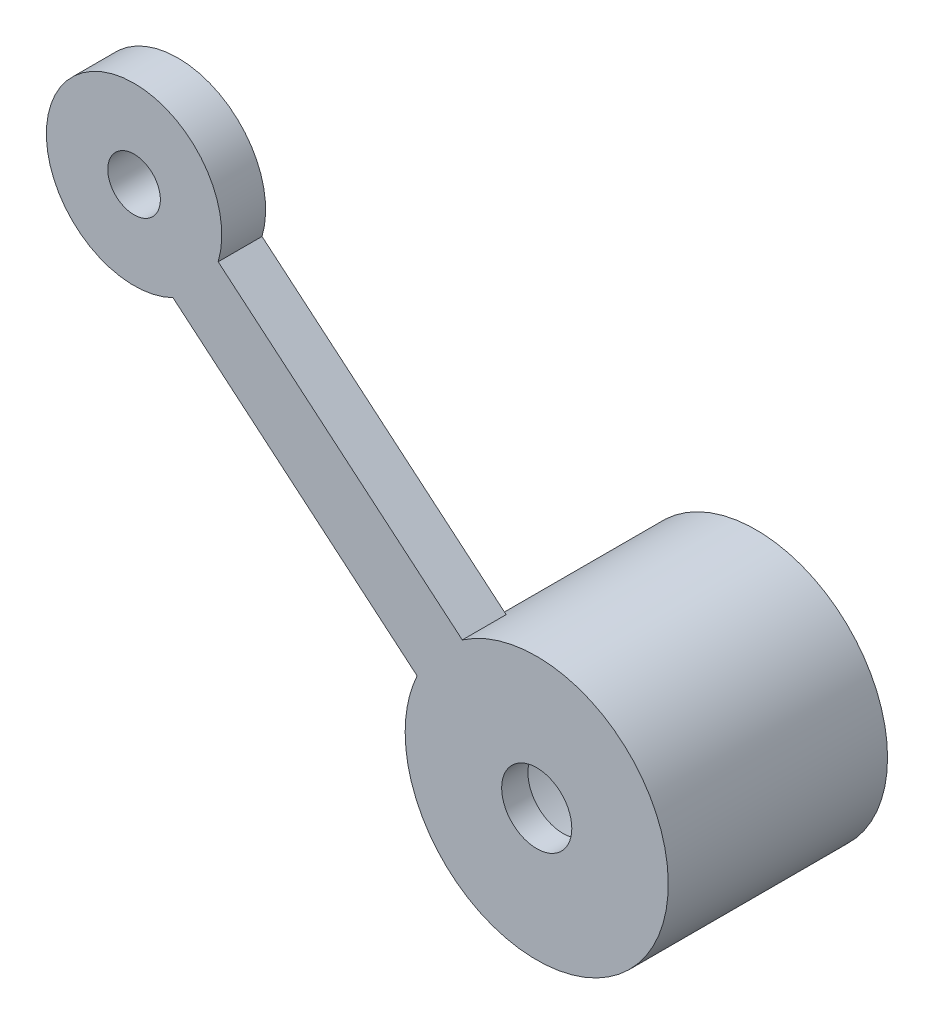
from build123d import *

# Parameters (mm, degrees)
SKETCH1_R           = 3
SKETCH1_R_2         = 4
BOSS_EXTRUDE1_DEPTH = 5
SKETCH2_R           = 13
CUT_EXTRUDE1_DEPTH  = 2
SKETCH4_R           = 1.25
BOSS_EXTRUDE2_DEPTH = 2
BOSS_EXTRUDE3_START = 20
SKETCH5_R           = 15
SKETCH5_R_2         = 13
BOSS_EXTRUDE3_DEPTH = 20


with BuildPart() as part:
    # Sketch1 → Boss-Extrude1 (new body)
    with BuildSketch(Plane.XY):
        with BuildLine():
            Line((4.437522393, -8.961495132), (32.27272364, -32.382887973))
            ThreePointArc((32.27272364, -32.382887973), (57.387408796, -48.287527496), (37.423393239, -26.261564368))
            Line((37.423393239, -26.261564368), (9.588191993, -2.840171527))
            ThreePointArc((9.588191993, -2.840171527), (-7.651654506, 6.438336999), (4.437522393, -8.961495132))
        make_face()
        Circle(SKETCH1_R, mode=Mode.SUBTRACT)
        with Locations((45.909927037, -38.630021997)):
            Circle(SKETCH1_R_2, mode=Mode.SUBTRACT)
    extrude(amount=BOSS_EXTRUDE1_DEPTH)

    # Sketch2 → Cut-Extrude1 (cut)
    with BuildSketch(Plane(origin=(0, 0, 0), x_dir=(-1, 0, 0), z_dir=(0, 0, -1))):
        with Locations((-45.909927037, -38.630021997)):
            Circle(SKETCH2_R)
    extrude(amount=-CUT_EXTRUDE1_DEPTH, mode=Mode.SUBTRACT)

    # Sketch4 → Boss-Extrude2 (add)
    with BuildSketch(Plane(origin=(0, 0, 0), x_dir=(-1, 0, 0), z_dir=(0, 0, -1))):
        with Locations((-45.909927037, -25.630021997)):
            Circle(SKETCH4_R)
        with Locations((-57.168257286, -45.130021997)):
            Circle(SKETCH4_R)
        with Locations((-34.651596788, -45.130021997)):
            Circle(SKETCH4_R)
    extrude(amount=-BOSS_EXTRUDE2_DEPTH)

    # Sketch5 → Boss-Extrude3 (add)
    with BuildSketch(Plane(origin=(0, 0, 0), x_dir=(-1, 0, 0), z_dir=(0, 0, -1)).offset(BOSS_EXTRUDE3_START)):
        with Locations((-45.909927037, -38.630021997)):
            Circle(SKETCH5_R)
        with Locations((-45.909927037, -38.630021997)):
            Circle(SKETCH5_R_2, mode=Mode.SUBTRACT)
    extrude(amount=-BOSS_EXTRUDE3_DEPTH)


solid = part.part
